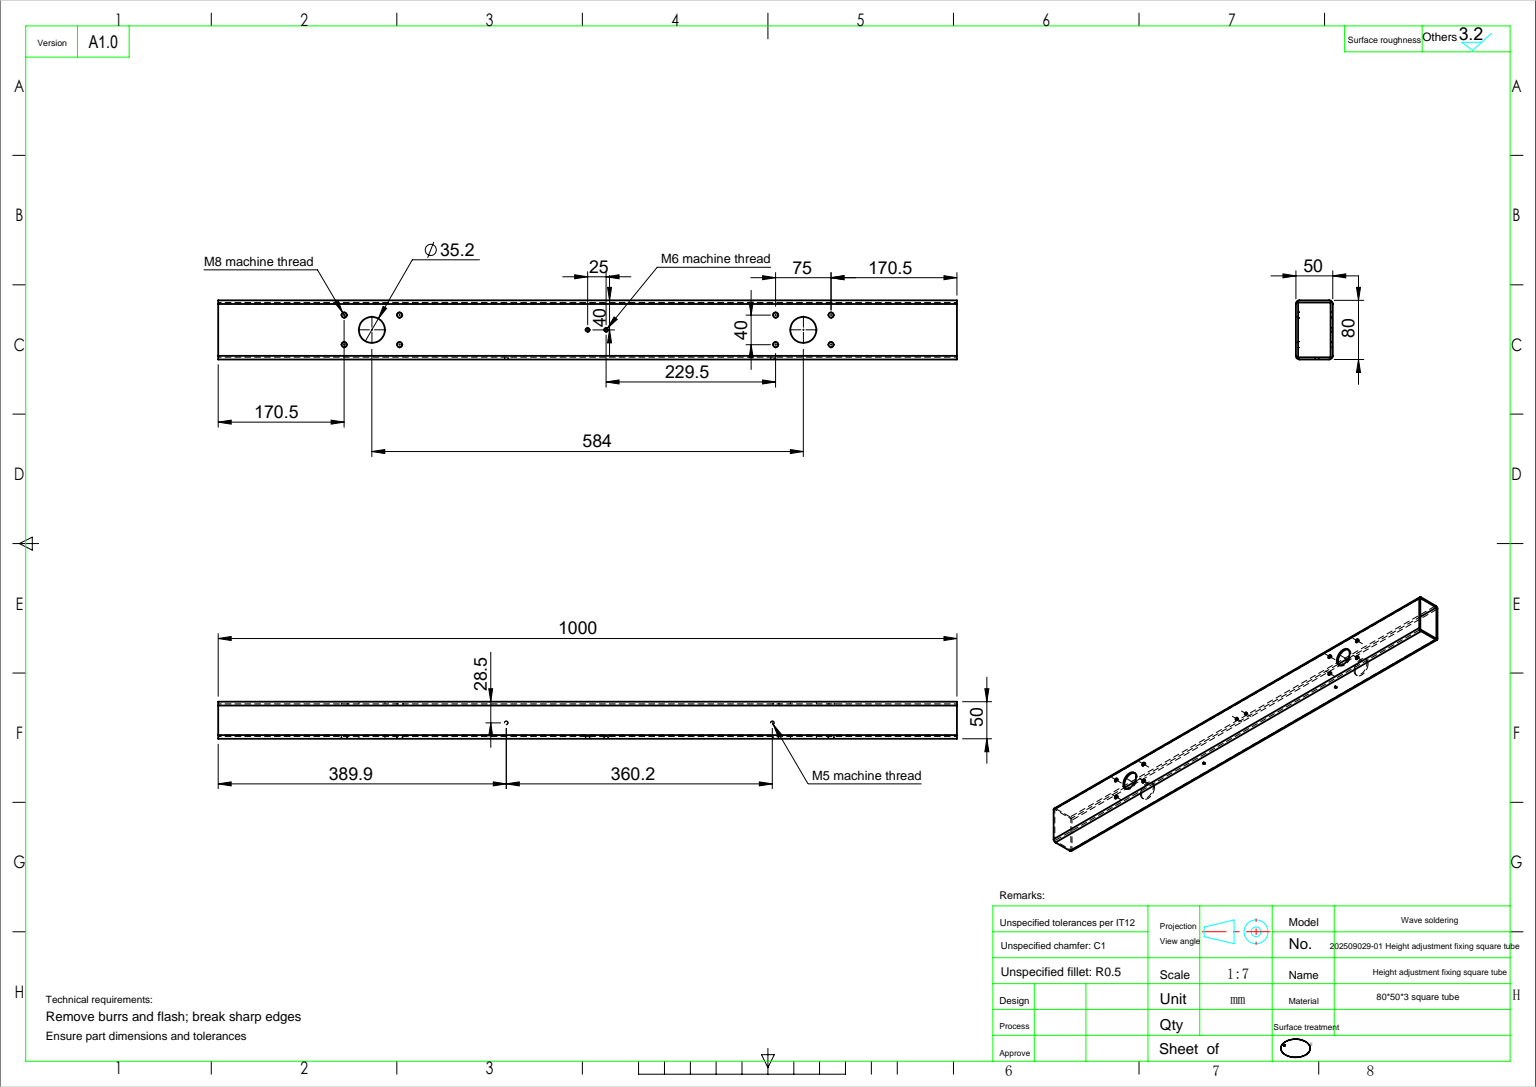
SolidWorks part; units mm, degrees
ref_plane "前视基准面" through (0, 0, 0) normal (0, 0, 1) x (1, 0, 0)
ref_plane "上视基准面" through (0, 0, 0) normal (0, 1, 0) x (1, 0, 0)
ref_plane "右视基准面" through (0, 0, 0) normal (1, 0, 0) x (0, 0, -1)
sketch "草图1" plane through (0, 0, 0) normal (0, 0, 1) x (1, 0, 0)
  line L1 (-500, 40) -> (500, 40)
  line L2 (-500, 40) -> (-500, -40)
  line L3 (-500, -40) -> (500, -40)
  line L4 (500, 40) -> (500, -40)
  line L5 (0, -40) -> (0, 40) construction
  line L6 (-500, 0) -> (500, 0) construction
  point P0 (0, 0)
  dimension "D1" = 1000
  dimension "D2" = 80
extrude "凸台-拉伸1" add sketch "草图1" along normal blind 50
shell "抽壳1" thickness 3
fillet "圆角1" radius 5 4 edges at (0, -40, 0) (0, -40, 50) (0, 40, 0) (0, 40, 50)
sketch "草图3" plane through (0, 0, 0) normal (0, 0, -1) x (-1, 0, 0)
  line L1 (-500, 40) -> (500, 40) construction
  line L2 (500, 35) -> (500, -35) construction
  circle A0 centre (-292, 0) radius 17.6
  circle A1 centre (292, 0) radius 17.6
  dimension "D1" = 35.2
  dimension "D2" = 584
  dimension "D3" = 208
  dimension "D4" = 40
extrude "切除-拉伸2" cut sketch "草图3" against normal through all
sketch "草图4" plane through (0, 0, 0) normal (0, 0, -1) x (-1, 0, 0)
  line L0 (500, -40) -> (-500, -40) construction
  line L3 (500, -40) -> (-500, -40) construction
  line L4 (-292, 0) -> (-309.7016, 0) construction
  line L5 (-292, 0) -> (-292, 46.6127) construction
  line L6 (292, 0) -> (267.0707, 0) construction
  line L7 (292, 0) -> (292, 47.5965) construction
  circle A0 centre (-329.5, 20) radius 3.4
  circle A1 centre (-329.5, -20) radius 3.4
  circle A2 centre (-254.5, 20) radius 3.4
  circle A3 centre (-254.5, -20) radius 3.4
  circle A4 centre (254.5, 20) radius 3.4
  circle A5 centre (254.5, -20) radius 3.4
  circle A6 centre (329.5, 20) radius 3.4
  circle A7 centre (329.5, -20) radius 3.4
  point P23 (0, 0)
  point P25 (0, 0)
  point P31 (0, 0)
  dimension "D1" = 6.8
  dimension "D2" = 75
  dimension "D3" = 40
  dimension "D7" = 75
  dimension "D8" = 40
  dimension "D9" = 20
  dimension "D4" = 20
extrude "切除-拉伸3" cut sketch "草图4" against normal blind 10
cosmetic thread "装饰螺纹线1" parameters "D2"=8
cosmetic thread "装饰螺纹线2" parameters "D2"=8
cosmetic thread "装饰螺纹线3" parameters "D2"=8
cosmetic thread "装饰螺纹线4" parameters "D2"=8
cosmetic thread "装饰螺纹线5" parameters "D2"=8
cosmetic thread "装饰螺纹线6" parameters "D2"=8
cosmetic thread "装饰螺纹线7" parameters "D2"=8
cosmetic thread "装饰螺纹线8" parameters "D2"=8
sketch "草图5" plane through (0, 0, 0) normal (0, 0, -1) x (-1, 0, 0)
  line L0 (-500, -35) -> (-500, 35) construction
  line L1 (-500, 40) -> (500, 40) construction
  circle A0 centre (0, 0) radius 2.5
  circle A1 centre (25, 0) radius 2.5
  dimension "D1" = 25
  dimension "D2" = 5
  dimension "D3" = 500
  dimension "D4" = 40
extrude "切除-拉伸4" cut sketch "草图5" against normal blind 10
cosmetic thread "装饰螺纹线9" parameters "D1"=2.9999, "D2"=6
cosmetic thread "装饰螺纹线10" parameters "D1"=2.9999, "D2"=6
sketch "草图6" plane through (0, -40, 0) normal (0, -1, 0) x (1, 0, 0)
  line L0 (500, 0) -> (-500, 0) construction
  line L1 (500, 45) -> (500, 5) construction
  circle A0 centre (110.1, 21.5) radius 2.1
  circle A1 centre (-250.1, 21.5) radius 2.1
  dimension "D1" = 4.2
  dimension "D3" = 360.2
  dimension "D2" = 21.5
  dimension "D4" = 389.9
extrude "切除-拉伸5" cut sketch "草图6" against normal blind 10
cosmetic thread "装饰螺纹线11" parameters "D2"=5
cosmetic thread "装饰螺纹线12" parameters "D2"=5
